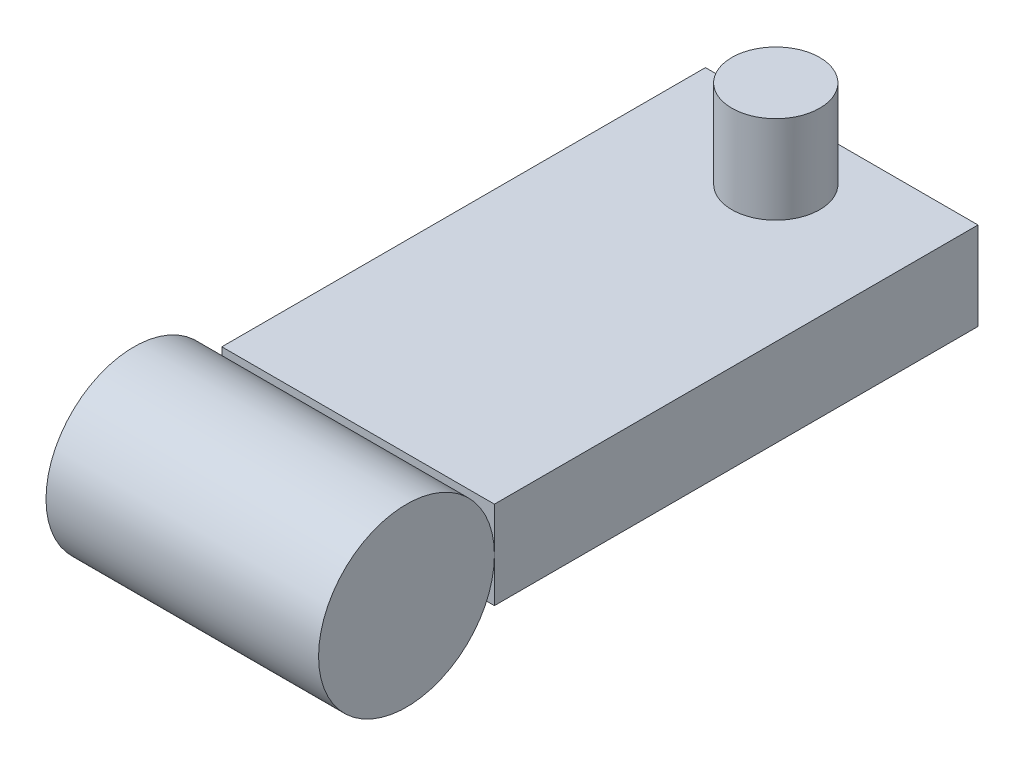
SolidWorks part; units mm, degrees
ref_plane "前视基准面" through (0, 0, 0) normal (0, 0, 1) x (1, 0, 0)
ref_plane "上视基准面" through (0, 0, 0) normal (0, 1, 0) x (1, 0, 0)
ref_plane "右视基准面" through (0, 0, 0) normal (1, 0, 0) x (0, 0, -1)
sketch "草图1" plane through (0, 0, 0) normal (0, 0, 1) x (1, 0, 0)
  line L1 (-31, -10) -> (31, -10)
  line L2 (-31, -10) -> (-31, 10)
  line L3 (-31, 10) -> (31, 10)
  line L4 (31, -10) -> (31, 10)
  line L5 (-31, -10) -> (31, 10) construction
  line L6 (-31, 10) -> (31, -10) construction
  point P0 (0, 0)
  dimension "D1" = 20
  dimension "D2" = 62
extrude "凸台-拉伸1" add sketch "草图1" along normal blind 110
sketch "草图2" plane through (31, 0, 0) normal (1, 0, 0) x (0, 0, -1)
  line L0 (-110, 0) -> (-147.5904, 0) construction
  line L1 (-110, -10) -> (-110, 10) construction
  circle A0 centre (-130, 0) radius 20
  dimension "D1" = 40
extrude "凸台-拉伸2" add sketch "草图2" against normal up to surface (62 mm away) separate body up to face at (-31, 0, 55)
sketch "草图3" plane through (0, 10, 0) normal (0, 1, 0) x (1, 0, 0)
  line L0 (0, 0) -> (0, -60.1133) construction
  line L1 (31, 0) -> (-31, 0) construction
  circle A0 centre (0, -15) radius 10
  dimension "D1" = 20
  dimension "D2" = 15
extrude "凸台-拉伸3" add sketch "草图3" along normal blind 20
